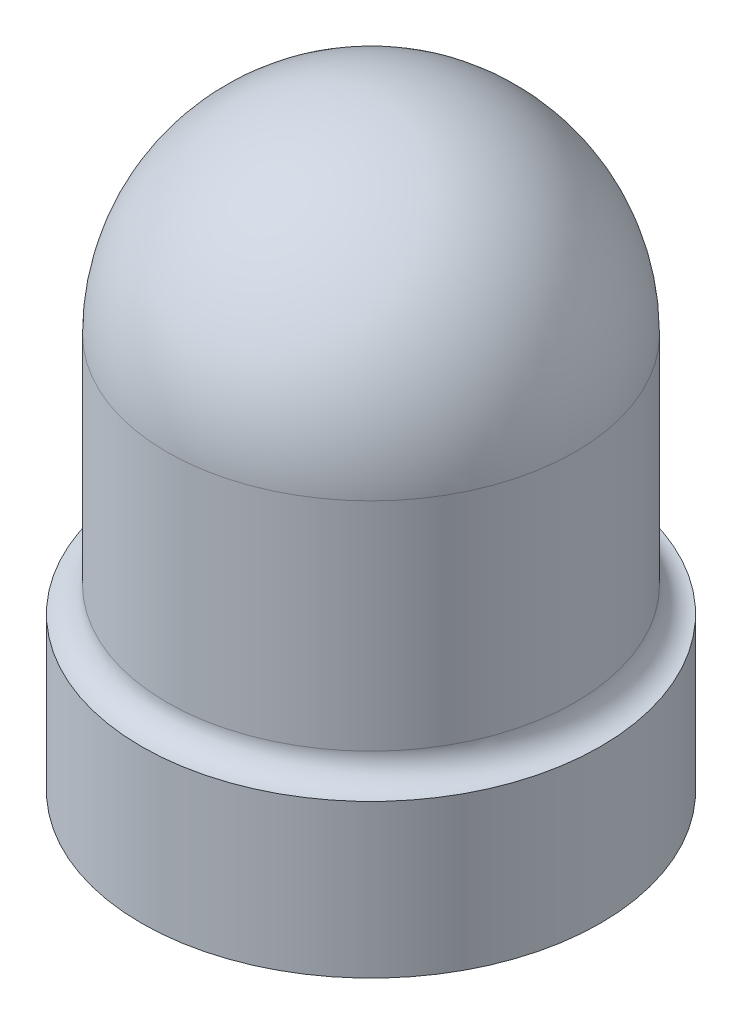
SolidWorks part; units mm, degrees
ref_plane "Front Plane" through (0, 0, 0) normal (0, 0, 1) x (1, 0, 0)
ref_plane "Top Plane" through (0, 0, 0) normal (0, 1, 0) x (1, 0, 0)
ref_plane "Right Plane" through (0, 0, 0) normal (1, 0, 0) x (0, 0, -1)
other "Configuration Table"
sketch "Sketch2" plane through (0, 0, 0) normal (0, 0, 1) x (1, 0, 0)
  line L0 (0, -51.943) -> (0, 51.943) construction
  line L1 (-16, 31) -> (-16, 14)
  line L2 (-13, 0) -> (-18, 0)
  line L3 (-18, 0) -> (-18, 12)
  line L4 (-13, 0) -> (-13, 15)
  line L5 (-12, 31) -> (-12, 15)
  line L6 (-12, 15) -> (-13, 15)
  line L7 (0, 47) -> (0, 43)
  arc A0 (0, 43) -> (-12, 31) centre (0, 31) ccw
  arc A1 (0, 47) -> (-16, 31) centre (0, 31) ccw
  arc A3 (-18, 12) -> (-16, 14) centre (-18, 14) ccw
  point P4 (0, 0)
  dimension "D1" = 32
  dimension "D2" = 24
  dimension "D6" = 4
  dimension "D3" = 31
  dimension "D4" = 18
  dimension "D5" = 12
  dimension "D7" = 13
  dimension "D8" = 15
revolve "Revolve1" add sketch "Sketch2" angle 360 about L0
sketch "Sketch3" plane through (0, 0, 0) normal (1, 0, 0) x (0, 0, -1)
  line L0 (-18, 0) -> (18, 0) construction
  circle A0 centre (0, 6) radius 2.5
  dimension "D1" = 5
  dimension "D2" = 6
extrude "Cut-Extrude1" cut sketch "Sketch3" against normal blind 40
chamfer "Chamfer1" distance 1.5 angle 45 1 edges at (13, 0, 0)
